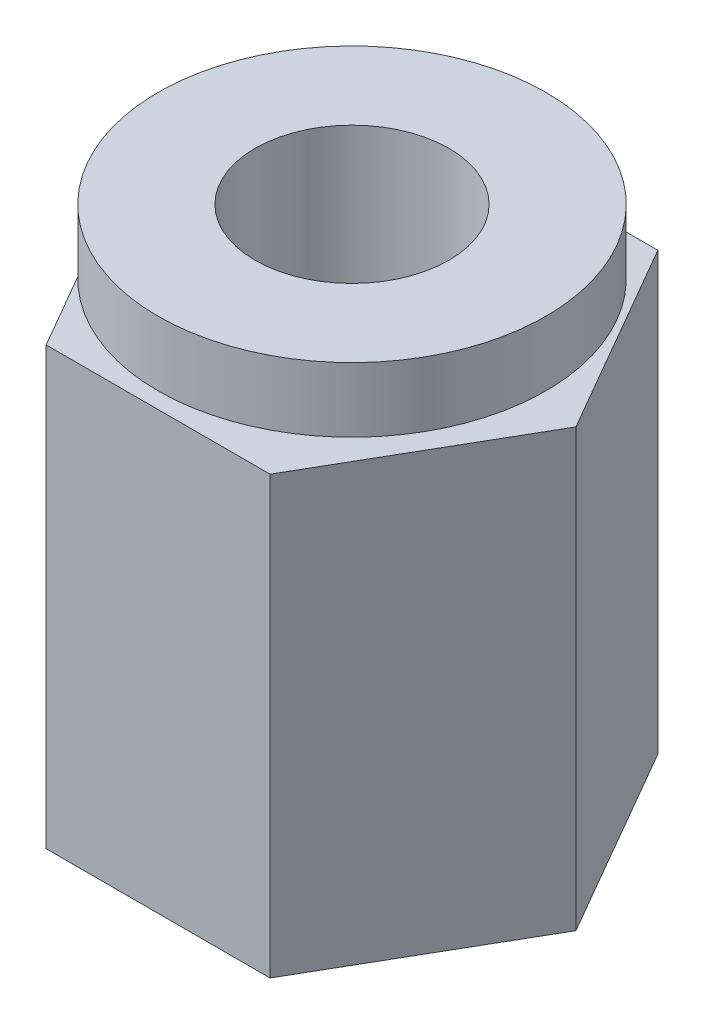
from build123d import *

# Parameters (mm, degrees)
BOSS_EXTRUDE1_DEPTH = 13.5
HOLE1_D             = 6


with BuildPart() as part:
    # Sketch1 → Boss-Extrude1 (new body)
    with BuildSketch(Plane(origin=(0, 0, 0), x_dir=(1, 0, 0), z_dir=(0, 1, 0))):
        Polygon((-6.92820323, 0), (-3.464101615, -6), (3.464101615, -6), (6.92820323, 0), (3.464101615, 6), (-3.464101615, 6), align=None)
    extrude(amount=BOSS_EXTRUDE1_DEPTH)

    # Sketch2 → Revolve1 (revolve)
    with BuildSketch(Plane.XY, mode=Mode.PRIVATE) as revolve1_sk:
        Polygon((0, 16), (6, 16), (6, 14), (5, 14), (5, 13.5), (0, 13.5), align=None)
    revolve(revolve1_sk.sketch.rotate(Axis((0, 13.5, 0), (0, 1, 0)), 270), axis=Axis((0, 13.5, 0), (0, 1, 0)))

    # Hole1 (through all)
    with Locations(Plane(origin=(0, 0, 0), x_dir=(-1, 0, 0), z_dir=(0, -1, 0))):
        with Locations((0, 0)):
            Hole(HOLE1_D / 2)


solid = part.part
